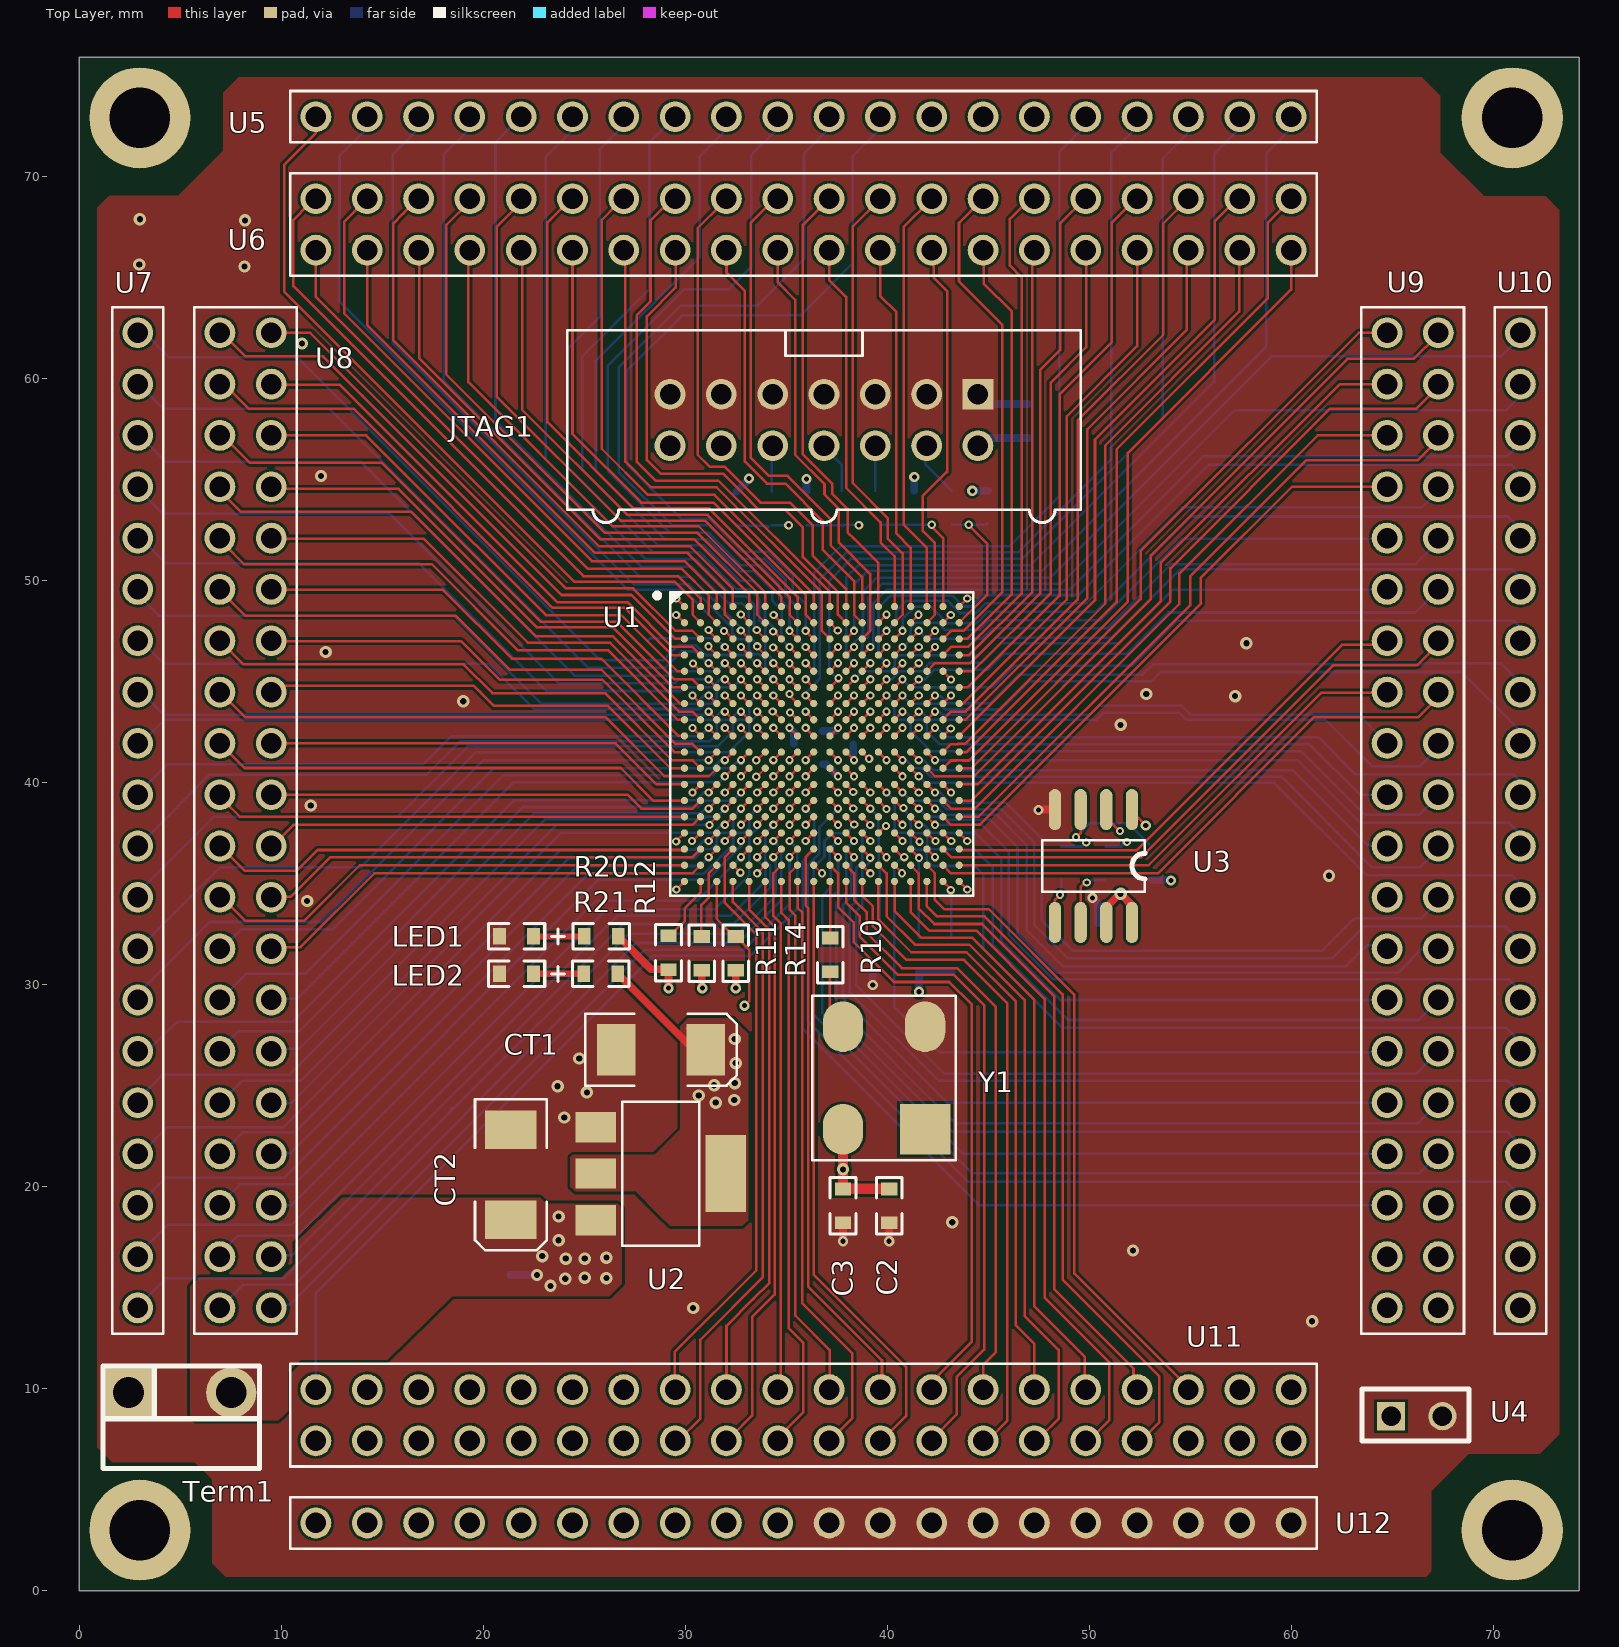
[diagram p0: Top Layer view]
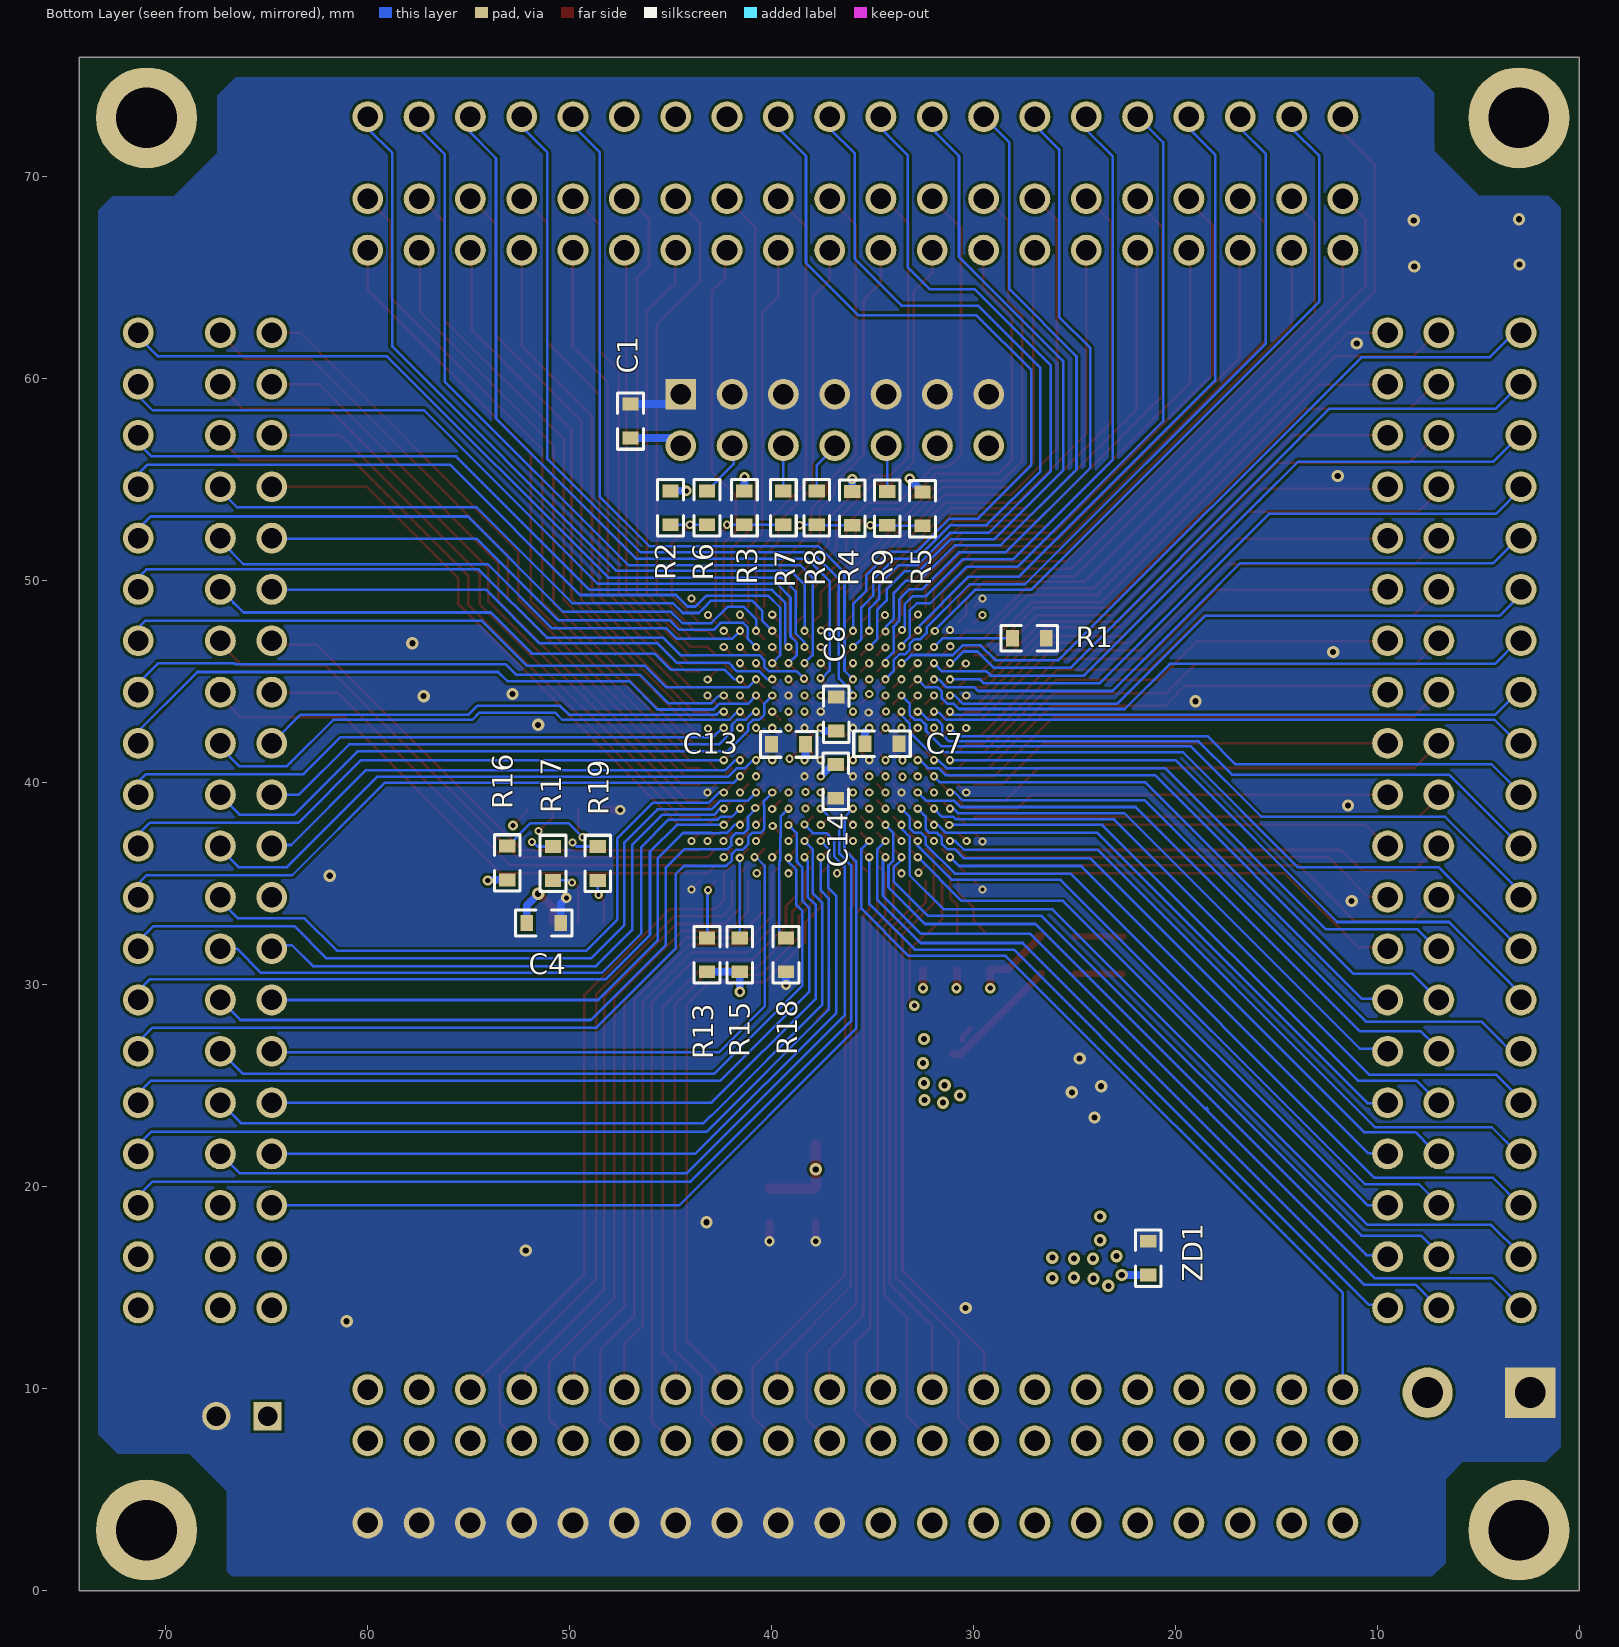
[diagram p1: Bottom Layer view, seen from below]
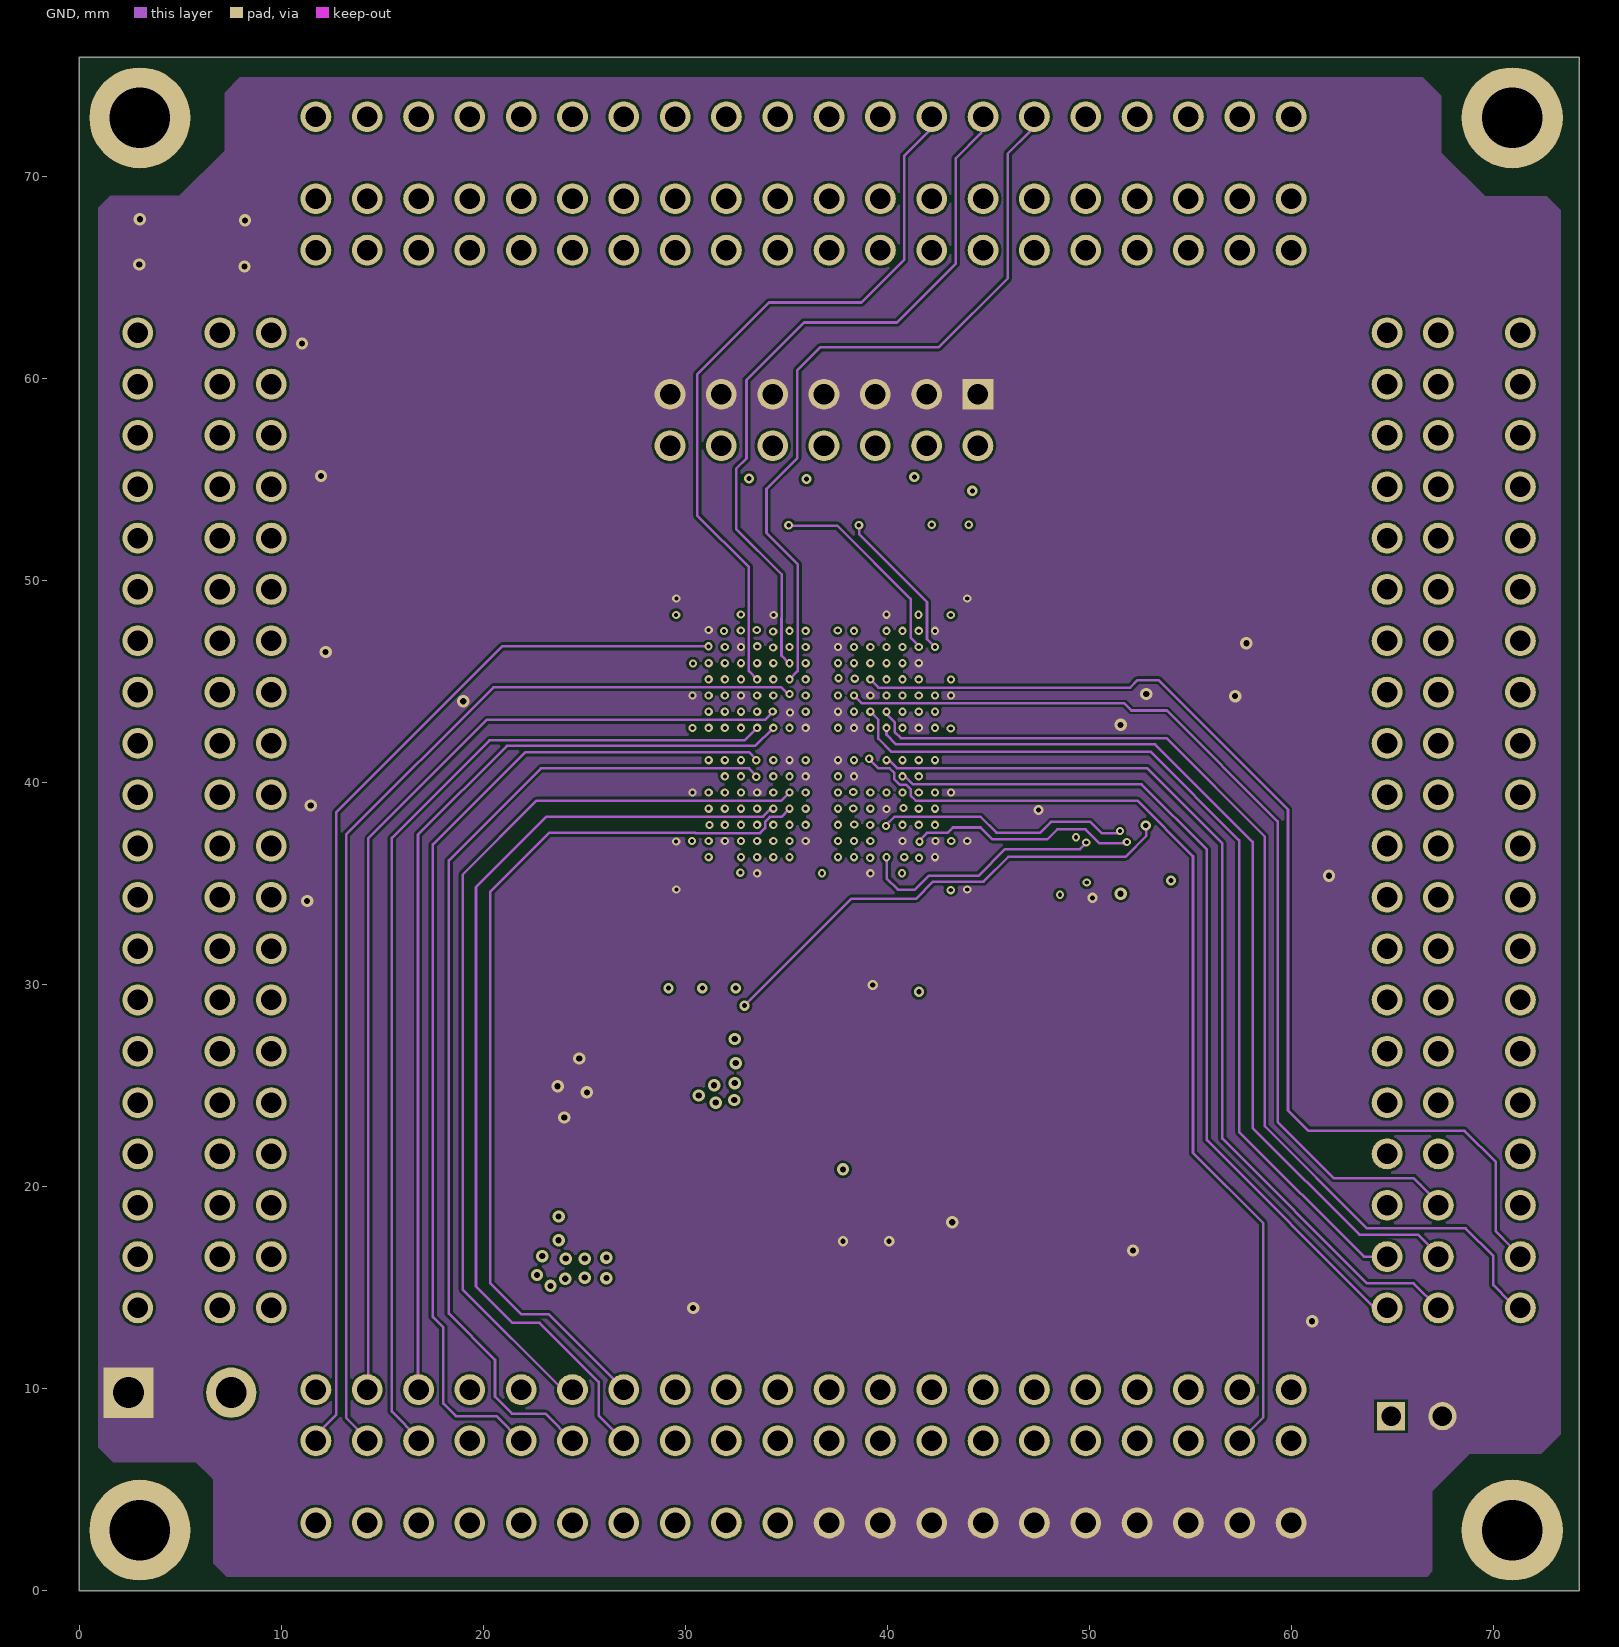
[diagram p2: GND]
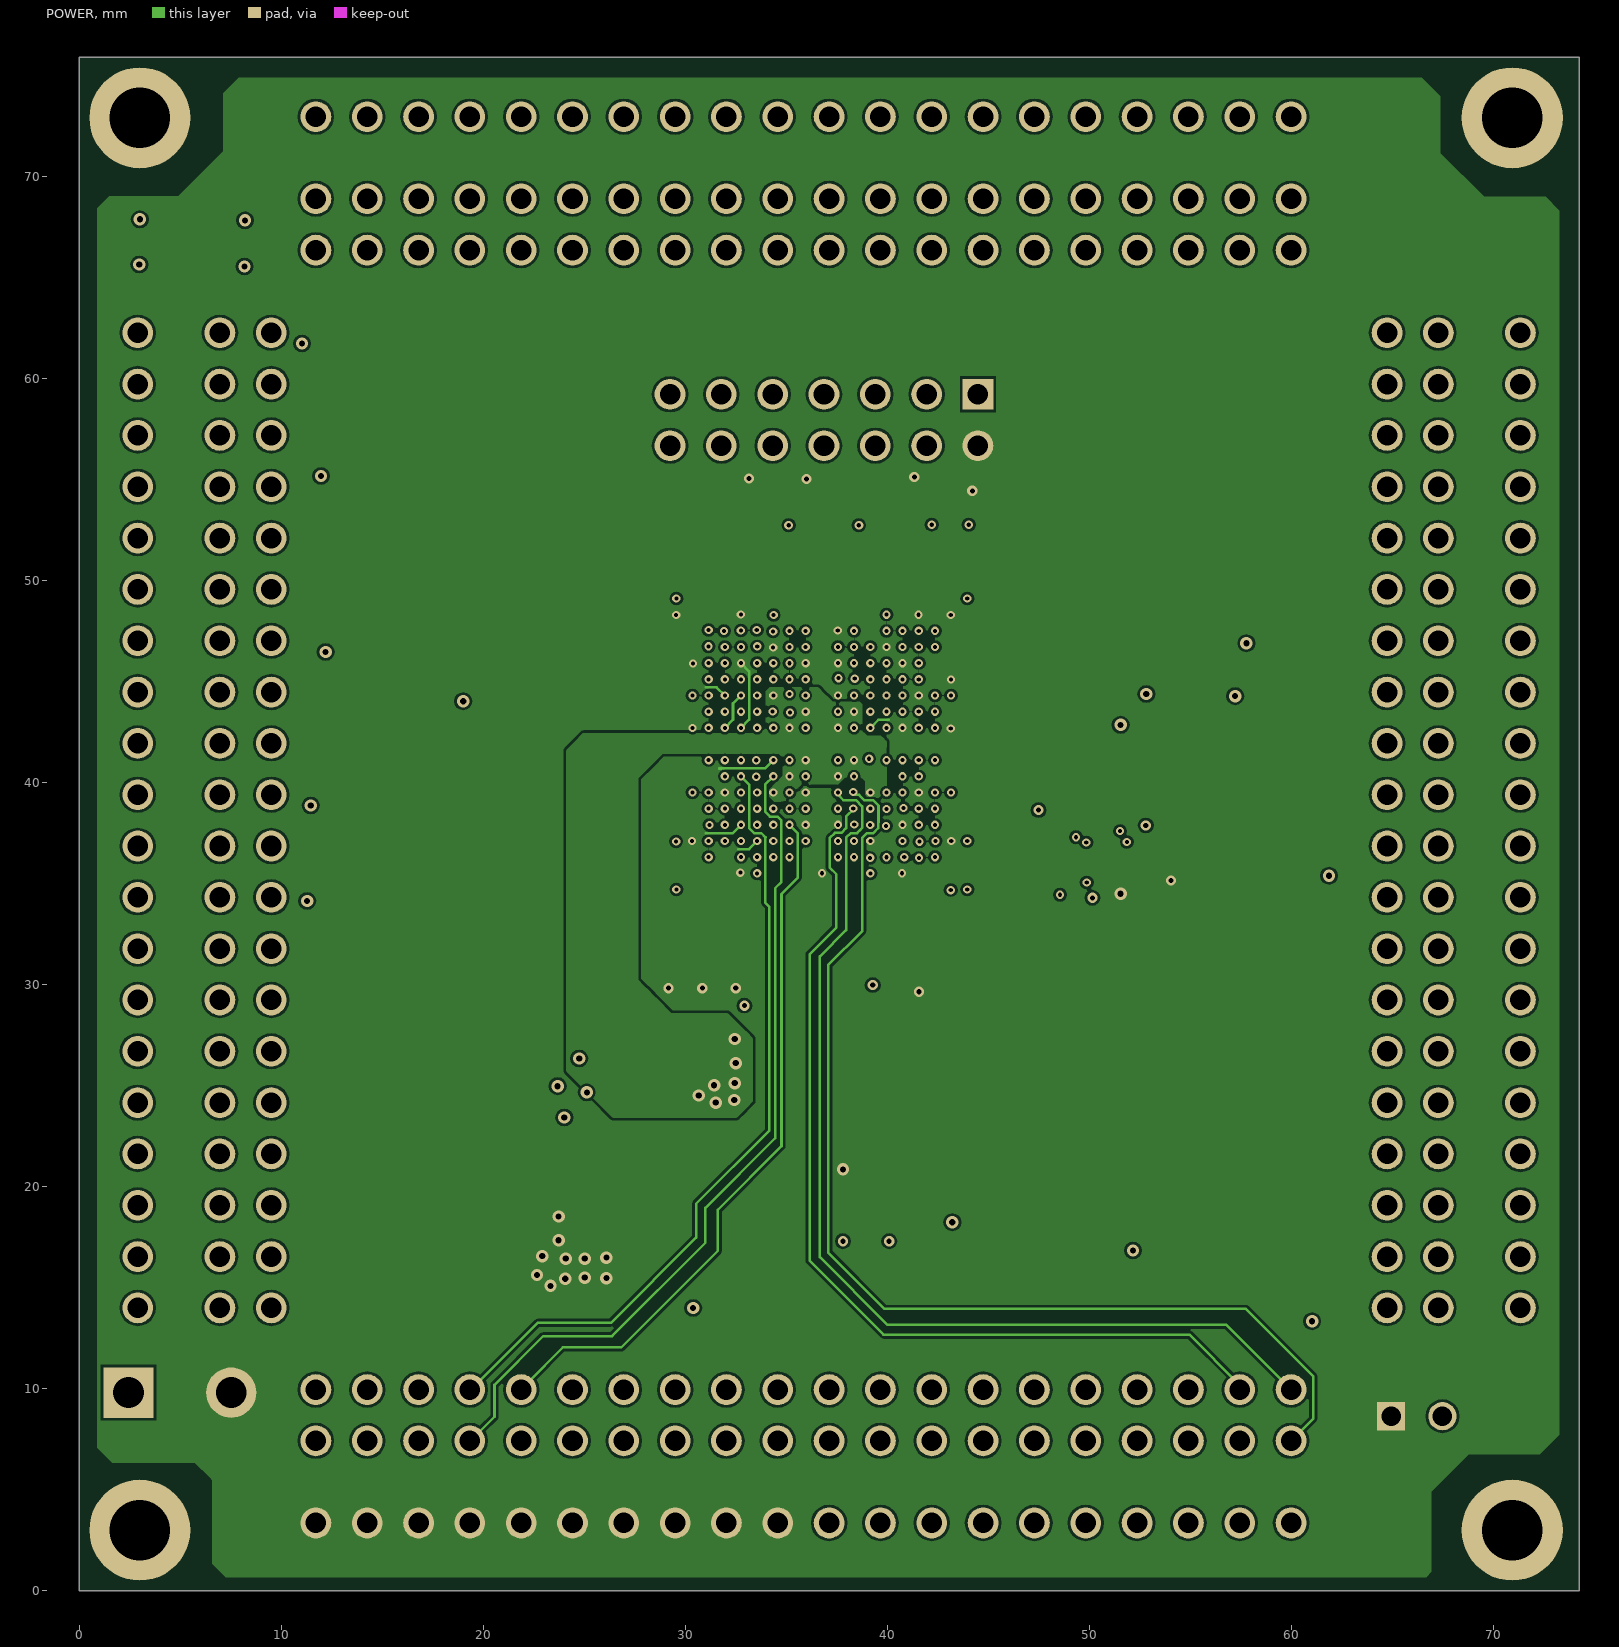
[diagram p3: POWER]
# Altium PCB MISC103828.PcbDoc (part 1 of 4)
Units mm, origin at the board's own origin, x right, y up, seen from the top; angles counter-clockwise.
Board outline 74.24 x 75.89 mm, 4 copper layers (Top Layer, GND, POWER, Bottom Layer); 49 components, 246 nets, 670 pads, 283 vias.

## Layer stack, top to bottom (the 12.6 mil dielectric is the usual default, probably not edited)
Top Layer: signal copper 0.0356
Dielectric: core 0.32, FR-4, Dk 4.8
GND: signal copper 0.0356
Dielectric: prepreg 0.32, FR-4, Dk 4.8
POWER: signal copper 0.0356
Dielectric: core 0.32, FR-4, Dk 4.8
Bottom Layer: signal copper 0.0356

## Board outline
0,0 0,75.889 74.244,75.889 74.244,0

## Design rules (kind name [scope] priority, off if disabled: settings)
Clearance [All] p1: gap=0.127
FabricationTestPointUsage TestPointUsage [All] p1: valid=0 allowmultiple=FALSE
FabricationTestpoint Testpoint [(IsPad And (OnTopLayer Or OnBottomLayer))] p1: side=3 testpointundercomponent=TRUE minsize=1.016 maxsize=2.54 preferedsize=1.524 minholesize=0 maxholesize=1.016 preferedholesize=0.813 testpointgrid=0.025 allowsidetop=TRUE allowsidebottom=TRUE usegrid=TRUE gridtolerance=0
HoleSize [All] p1: absolutevalues=TRUE maxlimit=12.7 minlimit=0.025 maxpercent=80.000 minpercent=20.000
HoleToHoleClearance [All] p1: gap=0.152 allowstackedmicrovias=TRUE
MinimumSolderMaskSliver [All] p1: minsoldermaskwidth=0.152
PolygonConnect PolygonConnect_1 [All vs isvia] p1: connectstyle=Direct reliefconductorwidth=0.254 reliefentries=4 polygonreliefangle="90 Angle"
PolygonConnect [All] p2: connectstyle=Direct reliefconductorwidth=0.254 reliefentries=4 polygonreliefangle="90 Angle"
RoutingVias [All] p1: holewidth=0.254 width=0.508 viastyle="Through Hole" minholewidth=0.203 minwidth=0.406 maxholewidth=0.508 maxwidth=0.762
SilkToSilkClearance [All] p1: silktosilkclearance=0
SilkscreenOverComponentPads [All] p1: minsilkscreentomaskgap=0
SolderMaskExpansion [All] p1: expansion=0.102
Width [All] p1: maxlimit=0.508 minlimit=0.127 preferedwidth=0.127 minimp=50.000000 maximp=50.000000 favimp=50.000000
21 further rules are at their usual default settings.

## Components (designator, comment, footprint, x,y, rotation, side; value= is the part's Value field where it differs from the comment)
C1 "0.1u" 0603 46.965,58.725 r270 bottom
C2 "0.1uF" 0603 40.081,18.212 r90 top
C3 "0.1uF" 0603 37.795,18.212 r90 top
C4 "0.1u" 0603 52.095,33.045 r180 bottom
C7 "0.1uF" 0603 33.68,41.91 r0 bottom
C8 "0.1uF" 0603 36.779,44.221 r270 bottom
C13 "0.1uF" 0603 39.98,41.885 r180 bottom
C14 "0.1uF" 0603 36.805,39.218 r90 bottom
CT1 "22u/10V" 7227 26.543,26.772 r0 top
CT2 "22u/10V" 7227 21.361,22.835 r270 top
JTAG1 "JTAG" IDC14S 44.475,59.207 r180 top
LED1 "LED" DIODE_2 22.479,32.385 r180 top
LED2 "LED" DIODE_2 22.479,30.531 r180 top
R1 "51" 0603 26.391,47.142 r0 bottom
R2 "10k" 0603 44.983,54.432 r270 bottom
R3 "10k" 0603 41.326,54.432 r270 bottom
R4 "10k" 0603 35.992,54.407 r270 bottom
R5 "10k" 0603 32.512,54.381 r270 bottom
R6 "51" 0603 43.18,52.756 r90 bottom
R7 "51" 0603 39.395,52.756 r90 bottom
R8 "51" 0603 37.744,52.756 r90 bottom
R9 "51" 0603 34.265,52.73 r90 bottom
R10 "22" 0603 37.16,30.632 r90 top
R11 "4.7k" 0603 30.81,30.709 r90 top
R12 "4.7k" 0603 29.159,30.734 r90 top
R13 "4.7k" 0603 43.18,30.632 r90 bottom
R14 "4.7k" 0603 32.487,30.709 r90 top
R15 "4.7k" 0603 41.554,30.632 r90 bottom
R16 "4.7k" 0603 53.061,36.855 r270 bottom
R17 "22" 0603 50.8,36.83 r270 bottom
R18 "22" 0603 39.268,30.632 r90 bottom
R19 "22" 0603 48.59,36.83 r270 bottom
R20 "2k" 0603 24.994,32.385 r0 top
R21 "2k" 0603 24.968,30.531 r0 top
Term1 "Phonix Connector 2p" PhonixCon2P 2.438,9.804 r0 top
U1 "XC6SLX9-CSG324" CSG324 36.747,41.903 r0 top
U2 "LM1117-1.2V" SOT223 25.552,22.936 r270 top
U3 "M25P80" M25P16_SO-8 52.095,38.659 r270 top
U4 "TP2" TP2 64.922,8.636 r0 top
U5 "TP20_2.54mm" TP20_2.54mm 11.709,72.949 r0 top
U6 "TP20*2_2.54mm" TP20*2_2.54mm 11.709,66.345 r0 top
U7 "TP20_2.54mm" TP20_2.54mm 2.896,62.255 r270 top
U8 "TP20*2_2.54mm" TP20*2_2.54mm 6.96,62.255 r270 top
U9 "TP20*2_2.54mm" TP20*2_2.54mm 64.719,62.255 r270 top
U10 "TP20_2.54mm" TP20_2.54mm 71.323,62.255 r270 top
U11 "TP20*2_2.54mm" TP20*2_2.54mm 11.709,7.417 r0 top
U12 "TP20_2.54mm" TP20_2.54mm 11.709,3.353 r0 top
Y1 "30MHz-3.3V" OSC-SO4 41.859,22.835 r90 top
ZD1 "T3V3S5" 0603 21.336,17.297 r270 bottom

## Footprints (in the part's own frame and the unit in brackets; to place one, negate y for a bottom-side part, rotate by r counter-clockwise, add the part's x,y. Pads: shape width x height; smd on the part's side, far side on the other; paste and mask are expansions set on the pad)
0603 [mil]
  rect 25x32 smd: 1(0,0) 2(66,0)
  silkscreen extent -22,-25 88,25
7227 [mil]
  rect 75x100 smd: 1(176,0) 2(1,0)
  silkscreen extent -59,-70 236,70
CSG324 [mm] "BGA, 324-Leads, Body 15x15mm, Pitch 0.8mm"
  round 0.36 smd: A1(-6.8,6.8) A2(-6,6.8) A3(-5.2,6.8) A4(-4.4,6.8) A5(-3.6,6.8) A6(-2.8,6.8) A7(-2,6.8) A8(-1.2,6.8) A9(-0.4,6.8) A10(0.4,6.8) A11(1.2,6.8) A12(2,6.8) A13(2.8,6.8) A14(3.6,6.8) A15(4.4,6.8) A16(5.2,6.8) A17(6,6.8) A18(6.8,6.8) B1(-6.8,6) B2(-6,6) B3(-5.2,6) B4(-4.4,6) B5(-3.6,6) B6(-2.8,6) B7(-2,6) B8(-1.2,6) B9(-0.4,6) B10(0.4,6) B11(1.2,6) B12(2,6) B13(2.8,6) B14(3.6,6) B15(4.4,6) B16(5.2,6) B17(6,6) B18(6.8,6) C1(-6.8,5.2) C2(-6,5.2) C3(-5.2,5.2) C4(-4.4,5.2) C5(-3.6,5.2) C6(-2.8,5.2) C7(-2,5.2) C8(-1.2,5.2) C9(-0.4,5.2) C10(0.4,5.2) C11(1.2,5.2) C12(2,5.2) C13(2.8,5.2) C14(3.6,5.2) C15(4.4,5.2) C16(5.2,5.2) C17(6,5.2) C18(6.8,5.2) D1(-6.8,4.4) D2(-6,4.4) D3(-5.2,4.4) D4(-4.4,4.4) D5(-3.6,4.4) D6(-2.8,4.4) D7(-2,4.4) D8(-1.2,4.4) D9(-0.4,4.4) D10(0.4,4.4) D11(1.2,4.4) D12(2,4.4) D13(2.8,4.4) D14(3.6,4.4) D15(4.4,4.4) D16(5.2,4.4) D17(6,4.4) D18(6.8,4.4) E1(-6.8,3.6) E2(-6,3.6) E3(-5.2,3.6) E4(-4.4,3.6) E5(-3.6,3.6) E6(-2.8,3.6) E7(-2,3.6) E8(-1.2,3.6) E9(-0.4,3.6) E10(0.4,3.6) E11(1.2,3.6) E12(2,3.6) E13(2.8,3.6) E14(3.6,3.6) E15(4.4,3.6) E16(5.2,3.6) E17(6,3.6) E18(6.8,3.6) F1(-6.8,2.8) F2(-6,2.8) F3(-5.2,2.8) F4(-4.4,2.8) F5(-3.6,2.8) F6(-2.8,2.8) F7(-2,2.8) F8(-1.2,2.8) F9(-0.4,2.8) F10(0.4,2.8) F11(1.2,2.8) F12(2,2.8) F13(2.8,2.8) F14(3.6,2.8) F15(4.4,2.8) F16(5.2,2.8) F17(6,2.8) F18(6.8,2.8) G1(-6.8,2) G2(-6,2) G3(-5.2,2) G4(-4.4,2) G5(-3.6,2) G6(-2.8,2) G7(-2,2) G8(-1.2,2) G9(-0.4,2) G10(0.4,2) G11(1.2,2) G12(2,2) G13(2.8,2) G14(3.6,2) G15(4.4,2) G16(5.2,2) G17(6,2) G18(6.8,2) H1(-6.8,1.2) H2(-6,1.2) H3(-5.2,1.2) H4(-4.4,1.2) H5(-3.6,1.2) H6(-2.8,1.2) H7(-2,1.2) H8(-1.2,1.2) H9(-0.4,1.2) H10(0.4,1.2) H11(1.2,1.2) H12(2,1.2) H13(2.8,1.2) H14(3.6,1.2) H15(4.4,1.2) H16(5.2,1.2) H17(6,1.2) H18(6.8,1.2) J1(-6.8,0.4) J2(-6,0.4) J3(-5.2,0.4) J4(-4.4,0.4) J5(-3.6,0.4) J6(-2.8,0.4) J7(-2,0.4) J8(-1.2,0.4) J9(-0.4,0.4) J10(0.4,0.4) J11(1.2,0.4) J12(2,0.4) J13(2.8,0.4) J14(3.6,0.4) J15(4.4,0.4) J16(5.2,0.4) J17(6,0.4) J18(6.8,0.4) K1(-6.8,-0.4) K2(-6,-0.4) K3(-5.2,-0.4) K4(-4.4,-0.4) K5(-3.6,-0.4) K6(-2.8,-0.4) K7(-2,-0.4) K8(-1.2,-0.4) K9(-0.4,-0.4) K10(0.4,-0.4) K11(1.2,-0.4) K12(2,-0.4) K13(2.8,-0.4) K14(3.6,-0.4) K15(4.4,-0.4) K16(5.2,-0.4) K17(6,-0.4) K18(6.8,-0.4) L1(-6.8,-1.2) L2(-6,-1.2) L3(-5.2,-1.2) L4(-4.4,-1.2) L5(-3.6,-1.2) L6(-2.8,-1.2) L7(-2,-1.2) L8(-1.2,-1.2) L9(-0.4,-1.2) L10(0.4,-1.2) L11(1.2,-1.2) L12(2,-1.2) L13(2.8,-1.2) L14(3.6,-1.2) L15(4.4,-1.2) L16(5.2,-1.2) L17(6,-1.2) L18(6.8,-1.2) M1(-6.8,-2) M2(-6,-2) M3(-5.2,-2) M4(-4.4,-2) M5(-3.6,-2) M6(-2.8,-2) M7(-2,-2) M8(-1.2,-2) M9(-0.4,-2) M10(0.4,-2) M11(1.2,-2) M12(2,-2) M13(2.8,-2) M14(3.6,-2) M15(4.4,-2) M16(5.2,-2) M17(6,-2) M18(6.8,-2) N1(-6.8,-2.8) N2(-6,-2.8) N3(-5.2,-2.8) N4(-4.4,-2.8) N5(-3.6,-2.8) N6(-2.8,-2.8) N7(-2,-2.8) N8(-1.2,-2.8) N9(-0.4,-2.8) N10(0.4,-2.8) N11(1.2,-2.8) N12(2,-2.8) N13(2.8,-2.8) N14(3.6,-2.8) N15(4.4,-2.8) N16(5.2,-2.8) N17(6,-2.8) N18(6.8,-2.8) P1(-6.8,-3.6) P2(-6,-3.6) P3(-5.2,-3.6) P4(-4.4,-3.6) P5(-3.6,-3.6) P6(-2.8,-3.6) P7(-2,-3.6) P8(-1.2,-3.6) P9(-0.4,-3.6) P10(0.4,-3.6) P11(1.2,-3.6) P12(2,-3.6) P13(2.8,-3.6) P14(3.6,-3.6) P15(4.4,-3.6) P16(5.2,-3.6) P17(6,-3.6) P18(6.8,-3.6) R1(-6.8,-4.4) R2(-6,-4.4) R3(-5.2,-4.4) R4(-4.4,-4.4) R5(-3.6,-4.4) R6(-2.8,-4.4) R7(-2,-4.4) R8(-1.2,-4.4) R9(-0.4,-4.4) R10(0.4,-4.4) R11(1.2,-4.4) R12(2,-4.4) R13(2.8,-4.4) R14(3.6,-4.4) R15(4.4,-4.4) R16(5.2,-4.4) R17(6,-4.4) R18(6.8,-4.4) T1(-6.8,-5.2) T2(-6,-5.2) T3(-5.2,-5.2) T4(-4.4,-5.2) T5(-3.6,-5.2) T6(-2.8,-5.2) T7(-2,-5.2) T8(-1.2,-5.2) T9(-0.4,-5.2) T10(0.4,-5.2) T11(1.2,-5.2) T12(2,-5.2) T13(2.8,-5.2) T14(3.6,-5.2) T15(4.4,-5.2) T16(5.2,-5.2) T17(6,-5.2) T18(6.8,-5.2) U1(-6.8,-6) U2(-6,-6) U3(-5.2,-6) U4(-4.4,-6) U5(-3.6,-6) U6(-2.8,-6) U7(-2,-6) U8(-1.2,-6) U9(-0.4,-6) U10(0.4,-6) U11(1.2,-6) U12(2,-6) U13(2.8,-6) U14(3.6,-6) U15(4.4,-6) U16(5.2,-6) U17(6,-6) U18(6.8,-6) V1(-6.8,-6.8) V2(-6,-6.8) V3(-5.2,-6.8) V4(-4.4,-6.8) V5(-3.6,-6.8) V6(-2.8,-6.8) V7(-2,-6.8) V8(-1.2,-6.8) V9(-0.4,-6.8) V10(0.4,-6.8) V11(1.2,-6.8) V12(2,-6.8) V13(2.8,-6.8) V14(3.6,-6.8) V15(4.4,-6.8) V16(5.2,-6.8) V17(6,-6.8) V18(6.8,-6.8)
  silkscreen extent -8.27,-7.5 7.5,7.5
DIODE_2 [mil]
  rect 25x32 smd: A(0,0) K(66,0)
  silkscreen extent -60,-25 88,25
IDC14S [mil]
  rect 60x60 hole 40: 1(0,0)
  round 60 hole 40: 2(0,100) 3(100,0) 4(100,100) 5(200,0) 6(200,100) 7(300,0) 8(300,100) 9(400,0) 10(400,100) 11(500,0) 12(500,100) 13(600,0) 14(600,100)
  silkscreen extent -200,-125 800,250
M25P16_SO-8 [mil]
  oval 80x24 smd: 1(0,0) 2(0,-50) 3(0,-100) 4(0,-150) 5(220,-150) 6(220,-100) 7(220,-50) 8(220,0)
  silkscreen extent 60,-175 160,25
OSC-SO4 [mm]
  rect 2.5x2.5 smd: 1(0,0)
  oval 2.5x2 smd: 2(5.08,0) 3(5.08,4.064) 4(0,4.064)
  silkscreen extent -1.52,-1.52 6.6,5.59
PhonixCon2P [mil]
  rect 98x98 hole 60: 1(0,0)
  round 98 hole 60: 2(200,0)
  silkscreen extent -50,-148 255,52
SOT223 [mil]
  rect 59x79 smd: 1(0,0) 2(90,0) 3(181,0)
  rect 150x79 smd: 2(90,254)
  silkscreen extent -49,52 231,202
TP2 [mil]
  rect 55x55 hole 38: 1(0,0)
  round 55 hole 38: 2(100,0)
  silkscreen extent -57,-48 152,53
TP20*2_2.54mm [mil]
  round 60 hole 40: 1(0,0) 2(0,100) 3(100,0) 4(100,100) 5(200,0) 6(200,100) 7(300,0) 8(300,100) 9(400,0) 10(400,100) 11(500,0) 12(500,100) 13(600,0) 14(600,100) 15(700,0) 16(700,100) 17(800,0) 18(800,100) 19(900,0) 20(900,100) 21(1000,0) 22(1000,100) 23(1100,0) 24(1100,100) 25(1200,0) 26(1200,100) 27(1300,0) 28(1300,100) 29(1400,0) 30(1400,100) 31(1500,0) 32(1500,100) 33(1600,0) 34(1600,100) 35(1700,0) 36(1700,100) 37(1800,0) 38(1800,100) 39(1900,0) 40(1900,100)
  silkscreen extent -50,-50 1950,150
TP20_2.54mm [mil]
  round 60 hole 40: 1(0,0) 2(100,0) 3(200,0) 4(300,0) 5(400,0) 6(500,0) 7(600,0) 8(700,0) 9(800,0) 10(900,0) 11(1000,0) 12(1100,0) 13(1200,0) 14(1300,0) 15(1400,0) 16(1500,0) 17(1600,0) 18(1700,0) 19(1800,0) 20(1900,0)
  silkscreen extent -50,-50 1950,50

## Part data
C1 C4: library part CAP, "Multilayer ceramic capacitor"
C2 C3 C7 C8 C13 C14: library part CAP, "Capacitor"
CT1 CT2: library part CAPACITOR, "Capacitor"
JTAG1: library part IDC14
R1 R2 R3 R4 R5 R6 R7 R8 R9 R10 R11 R12 R13 R14 R15 R16 R17 R18 R19 R20 R21: library part RES2
U1: library part XC6SLX25-CSG324
U2: library part 7810
Y1: library part OSCILLATOR
ZD1: library part "D Tunnel2", "Tunnel Diode - Dependent Source Model"

## Free pads (board coordinates)
  round 5 hole 3: 0(3,3) 0(3,72.889) 0(70.915,3) 0(70.915,72.889)

## Via types
v1: diameter 0.406, hole 0.203, Top Layer to Bottom Layer, 221 vias
v2: diameter 0.61, hole 0.305, Top Layer to Bottom Layer, 43 vias
v3: diameter 0.508, hole 0.254, Top Layer to Bottom Layer, 16 vias
v4: diameter 0.432, hole 0.229, Top Layer to Bottom Layer, 3 vias

## Nets (pads, with @x,y where several pads share a name; then routed paths per layer and width w, separated by ;. In a path a pad name is that pad's centre, name@x,y a point inside that pad or via, vN(x,y) a via of type N, cw(c..) or ccw(c..) an arc to the next point about the centre after c; other vN are vias at no path point)
+1.2V: C7.2 C8.2 C13.2 C14.2 CT1.1 R21.2 U1.G7 U1.H9 U1.H11 U1.J8 U1.J10 U1.K9 U1.K11 U1.L8 U1.L10 U1.M7 U1.M12 U2.2 | length 16.5
  Top Layer w0.127: v1(34.347,39.503) U1.M7@34.747,39.903 ; v1(34.347,44.303) U1.G7@34.747,43.903 ; v1(35.147,40.303) U1.L8@35.547,40.703 ; v1(35.147,42.703) U1.J8@35.547,42.303 ; v1(35.947,41.103) U1.K9@36.347,41.503 ; v1(35.947,43.503) U1.H9@36.347,43.103 ; U1.L10@37.147,40.703 v1(37.547,40.303) ; U1.J10@37.147,42.303 v1(37.547,42.703) ; U1.K11@37.947,41.503 v1(38.347,41.103) ; U1.H11@37.947,43.103 v1(38.347,43.503) ; U1.M12@38.747,39.903 v1(39.147,39.503)
  Top Layer w0.254: CT1.1@30.137,27.826 30.531,27.432 CT1.1@30.531,27.229
  Top Layer w0.381: R21.2@26.645,30.531 30.632,26.543 CT1.1@31.013,26.543
  Bottom Layer w0.381: v1(35.147,42.703) 35.357,42.494 C7.2@35.357,41.91 ; C8.2@36.779,42.545 37.389,42.545 v1(37.547,42.703) ; C14.2@36.805,40.894 36.957,40.894 v1(37.547,40.303) ; C13.2@38.303,41.885 38.303,41.148 v1(38.347,41.103)
  other v2: 31.496,24.155 32.41,24.282 30.658,24.511 31.42,25.019 32.436,25.121 32.487,26.111 32.436,27.305
+3.3V: C1.2 C2.2 C3.2 C4.1 CT2.1 JTAG1.2 R2.1 R3.1 R4.1 R5.1 R11.1 R12.1 R13.1 R14.1 R15.1 R16.2 R20.2 Term1.2 U1.B1 U1.B5 U1.B10 U1.B15 U1.B17 U1.D7 U1.D13 U1.E2 U1.E5 U1.E9 U1.E10 U1.E14 U1.E17 U1.G4 U1.G10 U1.G15 U1.J2 U1.J5 U1.J12 U1.J14 U1.J17 U1.K7 U1.M4 U1.M9 U1.M15 U1.P5 U1.P9 U1.P10 U1.P14 U1.R2 U1.R6 U1.R12 U1.R17 U1.U4 U1.U9 U1.U14 U2.3 U3.7 U3.8 U4.1 U12.1 U12.2 U12.3 U12.4 U12.5 U12.6 U12.7 U12.8 U12.9 U12.10 Y1.4 ZD1.2 | length 57.4
  Top Layer w0.127: v1(29.54,48.285) 29.565,48.285 U1.B1@29.947,47.903 ; v1(30.328,37.109) 30.347,37.109 30.363,37.125 30.369,37.125 U1.R2@30.747,37.503 ; v1(30.353,42.697) U1.J2@30.747,42.303 ; v1(30.369,45.888) 30.369,45.882 U1.E2@30.747,45.503 ; v1(31.947,39.503) U1.M4@32.347,39.903 ; v1(31.947,44.303) U1.G4@32.347,43.903 ; U1.U4@32.347,35.903 v1(32.715,35.535) ; v1(32.741,48.311) 32.766,48.285 U1.B5@33.147,47.903 ; v1(32.747,37.903) U1.P5@33.147,38.303 ; v1(32.747,42.703) U1.J5@33.147,42.303 ; v1(32.747,45.903) U1.E5@33.147,45.503 ; v1(33.547,37.103) U1.R6@33.947,37.503 ; v1(34.347,41.103) U1.K7@34.747,41.503 ; v1@34.468,46.609 34.747,46.329 U1.D7@34.747,46.303 ; v1(35.947,37.903) U1.P9@36.347,38.303 ; v1(35.947,39.503) U1.M9@36.347,39.903 ; v1(35.947,45.903) U1.E9@36.347,45.503 ; U1.U9@36.347,35.903 36.744,35.506 v1(36.751,35.506) ; U1.P10@37.147,38.303 v1(37.547,37.903) ; U1.G10@37.147,43.903 v1(37.547,44.303) ; U1.E10@37.147,45.503 v1(37.547,45.903) ; U1.B10@37.147,47.903 37.531,47.52 v1(37.538,47.52) ; U1.R12@38.747,37.503 v1(39.147,37.103) ; U1.J12@38.747,42.303 v1(39.147,42.703) ; U1.D13@39.547,46.303 v1(39.947,46.703) ; U1.U14@40.347,35.903 40.716,35.535 v1(40.716,35.509) ; U1.P14@40.347,38.303 v1(40.747,37.903) ; U1.J14@40.347,42.303 v1(40.747,42.703) ; U1.E14@40.347,45.503 v1(40.747,45.903) ; U1.M15@41.147,39.903 v1(41.547,39.503) ; U1.G15@41.147,43.903 v1(41.547,44.303) ; U1.B15@41.147,47.903 41.539,48.295 v1(41.539,48.301) ; U1.R17@42.747,37.503 43.145,37.106 v1(43.151,37.106) ; U1.J17@42.747,42.303 43.119,42.675 v1(43.126,42.675) ; U1.E17@42.747,45.503 43.144,45.107 v1(43.144,45.1) ; U1.B17@42.747,47.903 v1(43.129,48.285)
  Top Layer w0.381: R20.2@26.797,32.385 R20.2@26.67,32.385 28.296,30.759 R12.1@29.159,30.759 ; v3(29.159,29.82) R12.1@29.159,30.734 ; R11.1@30.81,30.709 30.81,29.82 v3(30.836,29.82) ; v3(32.487,29.82) R14.1@32.487,30.709 ; C3.2@37.795,19.964 C3.2@37.871,19.888 ; U3.7@50.825,33.071 50.825,33.833 v2@51.486,34.493 ; v2(51.537,34.493) 52.095,33.934 U3.8@52.095,33.071
  Top Layer w0.508: C3.2@37.795,19.964 Y1.4@37.795,22.073 ; C3.2@37.871,19.888 C2.2@40.081,19.888
  POWER w0.127: 31.013,37.497 32.341,37.497 v1(32.747,37.903) ; 31.013,44.704 31.547,44.704 v1(31.947,44.303) ; 31.674,40.691 31.778,40.691 31.784,40.697 33.941,40.697 v1(34.347,41.103) ; 32.614,36.703 33.147,36.703 v1(33.547,37.103) ; v1(32.747,42.703) 33.154,43.11 33.154,44.983 ; v1(32.747,45.903) 33.154,45.497 33.154,44.983 ; 33.154,45.11 33.154,44.983 ; v1(39.147,42.703) 39.548,43.104 40.056,43.104
  Bottom Layer w0.127: v1@30.328,42.697 v1(30.353,42.697) ; v1@32.715,48.235 32.766,48.285 v1(32.741,48.311) ; v1@43.129,45.085 v1(43.144,45.1)
  Bottom Layer w0.381: ZD1.2@21.336,15.621 v2@22.479,15.621 ; R5.1@32.512,54.381 33.147,55.016 v3(33.147,55.042) ; R4.1@35.992,54.407 v3(35.992,55.016) ; R3.1@41.326,54.432 v3(41.326,55.118) ; v3(41.554,29.642) R15.1@41.554,30.632 ; R15.1@41.758,30.582 41.808,30.632 R13.1@43.18,30.632 ; v3(44.196,54.432) R2.1@44.983,54.432 ; JTAG1.2@44.552,56.667 44.933,57.048 C1.2@46.965,57.048 ; v2@51.562,34.442 52.095,33.909 C4.1@52.095,33.045 ; R16.2@53.061,35.179 54,35.179 v3(54.026,35.154)
  other v1: 34.341,46.685
  other v2: 23.317,15.088 24.054,15.443 26.086,15.469 25.019,15.494 22.657,15.621 24.079,16.434 25.019,16.434 26.086,16.485 22.911,16.561 23.724,17.348 23.724,18.517 37.795,20.853
F_A2: U1.A2 U6.2 | length 31.6
  Top Layer w0.127: U6.2@11.659,68.605 11.354,68.605 10.592,67.843 10.592,64.567 24.943,50.216 29.642,50.216 30.747,49.11 U1.A2@30.747,48.703
F_A3: U1.A3 U6.4 | length 31.1
  Top Layer w0.127: U6.4@14.211,68.923 U6.4@14.275,68.986 ; U6.4@14.249,68.885 13.106,67.742 13.106,63.221 25.375,50.952 29.947,50.952 31.547,49.352 U1.A3@31.547,48.703
F_A4: U1.A4 U6.6 | length 30.3
  Top Layer w0.127: 16.078,68.199 16.027,68.148 ; U6.6@16.688,68.885 16.688,68.809 16.027,68.148 ; U1.A4@32.347,48.703 32.347,49.568 30.226,51.689 25.73,51.689 15.545,61.874 15.545,67.666 16.027,68.148
F_A5: U1.A5 U6.5 | length 27.1
  Top Layer w0.127: U6.5@16.789,66.345 16.815,66.319 16.815,61.011 25.781,52.045 30.429,52.045 33.147,49.326 U1.A5@33.147,48.703
F_A6: U1.A6 U6.7 | length 26
  Top Layer w0.127: U6.7@19.38,66.04 19.253,65.913 19.253,59.817 26.391,52.68 30.658,52.68 33.947,49.39 U1.A6@33.947,48.703
F_A7: U1.A7 U6.10 | length 28.7
  Top Layer w0.127: U6.10@21.844,68.656 21.819,68.656 20.65,67.488 20.65,59.106 26.797,52.959 30.963,52.959 34.747,49.174 U1.A7@34.747,48.703
F_A8: U1.A8 U6.12 | length 28.1
  Top Layer w0.127: U6.12@24.409,68.885 24.333,68.885 23.165,67.716 23.165,57.836 27.432,53.569 31.166,53.569 35.547,49.187 U1.A8@35.547,48.703
F_A9: U1.A9 U6.14 | length 26.5
  Top Layer w0.127: U6.14@26.619,68.631 26.619,68.605 25.857,67.843 25.857,56.515 28.143,54.229 31.445,54.229 36.347,49.327 U1.A9@36.347,48.703
F_A10: U1.A10 U6.16 | length 26.5
  Top Layer w0.127: U6.16@29.235,68.758 29.21,68.758 28.27,67.818 28.27,63.805 27.584,63.119 27.584,55.88 28.524,54.94 31.623,54.94 37.147,49.416 U1.A10@37.147,48.703
F_A11: U1.A11 U6.18 | length 24.8
  Top Layer w0.127: U6.18@31.826,68.656 30.607,67.437 30.607,56.21 31.191,55.626 31.934,55.626 33.712,53.848 35.179,53.848 36.297,52.73 36.297,51.232 37.947,49.581 U1.A11@37.947,48.703
F_A12: U1.A12 U6.20 | length 23.4
  Top Layer w0.127: U6.20@34.341,68.859 34.341,68.809 33.223,67.691 33.223,56.083 34.138,55.169 35.052,55.169 37.186,53.035 37.186,51.74 38.747,50.178 U1.A12@38.747,48.703
F_A13: U1.A13 U6.22 | length 22.4
  Top Layer w0.127: U6.22@37.109,68.885 35.814,67.589 35.814,56.236 37.262,54.788 37.262,54.305 38.024,53.543 38.024,52.375 38.354,52.045 ; 38.291,52.108 38.354,52.045 ; U1.A13@39.547,48.703 39.547,50.851 38.354,52.045
F_A14: U1.A14 U6.21 | length 19
  Top Layer w0.127: U6.21@37.109,66.345 37.109,64.872 37.948,64.033 37.948,54.585 39.662,52.87 39.662,51.88 40.347,51.194 U1.A14@40.347,48.703
F_A15: U1.A15 U6.23 | length 18.3
  Top Layer w0.127: U6.23@39.649,66.345 39.649,64.059 40.437,63.271 40.437,52.324 41.147,51.613 U1.A15@41.147,48.703
F_A16: U1.A16 U6.26 | length 21.2
  Top Layer w0.127: U1.A16@41.947,48.703 41.947,51.601 40.792,52.756 40.792,67.488 U6.26@42.189,68.885
F_B2: U1.B2 U5.1 | length 37.2
  Top Layer w0.127: U5.1@11.709,72.949 11.709,72.136 10.135,70.561 10.135,64.287 24.486,49.936 29.464,49.936 30.352,49.049 30.352,48.299 U1.B2@30.747,47.903
F_B3: U1.B3 U6.1 | length 29.4
  Top Layer w0.127: U6.1@11.709,66.345 11.709,64.033 25.171,50.571 29.82,50.571 31.152,49.239 31.152,48.299 U1.B3@31.547,47.903
F_B4: U1.B4 U6.3 | length 28.2
  Top Layer w0.127: U6.3@14.275,65.938 14.249,65.913 14.249,62.636 25.527,51.359 30.099,51.359 31.952,49.506 31.952,48.299 U1.B4@32.347,47.903
F_B6: U1.B6 U6.8 | length 30.7
  Top Layer w0.127: U6.8@19.329,68.885 19.329,68.758 18.161,67.589 18.161,60.198 26.01,52.349 30.593,52.349 33.553,49.389 33.553,48.87 33.552,48.868 33.552,48.299 U1.B6@33.947,47.903
F_B8: U1.B8 U6.9 | length 26.4
  Top Layer w0.127: 21.92,65.253 21.92,65.176 ; U6.9@21.996,66.243 21.92,66.167 21.92,65.176 ; U1.B8@35.547,47.903 35.152,48.299 35.152,49.188 31.101,53.238 27.127,53.238 21.92,58.445 21.92,65.176
F_B9: U1.B9 U6.11 | length 25.5
  Top Layer w0.127: U6.11@24.409,66.345 24.409,57.252 27.813,53.848 31.394,53.848 35.943,49.299 35.943,48.307 U1.B9@36.347,47.903
F_B11: U1.B11 U6.15 | length 25.4
  Top Layer w0.127: U6.15@29.566,65.964 29.515,65.913 29.515,64.491 28.092,63.068 28.092,55.956 28.778,55.27 31.877,55.27 33.198,53.95 ; 33.172,53.95 33.604,53.518 34.925,53.518 35.814,52.629 35.814,51.156 37.543,49.426 37.543,48.307 U1.B11@37.947,47.903
F_B12: U1.B12 U6.17 | length 22.8
  Top Layer w0.127: U6.17@31.979,65.862 32.055,65.938 32.055,66.548 32.029,66.573 32.029,65.227 32.944,64.313 32.944,60.833 ; 32.944,60.909 32.944,60.833 ; U1.B12@38.747,47.903 38.351,48.299 38.351,49.964 36.792,51.524 36.792,52.946 34.95,54.788 34.036,54.788 32.944,55.88 32.944,60.833
F_B14: U1.B14 U6.24 | length 22.7
  Top Layer w0.127: U6.24@39.649,68.885 38.278,67.513 38.278,54.813 40.005,53.086 40.005,52.07 40.743,51.332 40.743,48.299 U1.B14@40.347,47.903
F_B16: U1.B16 U6.25 | length 20.8
  Top Layer w0.127: U1.B16@41.947,47.903 42.343,48.299 42.343,51.84 41.745,52.438 41.745,54.191 42.901,55.347 ; U6.25@42.113,65.862 42.139,65.888 42.139,66.523 42.291,66.675 42.291,64.973 42.951,64.313 42.951,55.347
F_C1: U1.C1 U8.1 | length 28.9
  Top Layer w0.127: U8.1@7.264,62.052 8.23,61.087 12.065,61.087 14.021,59.131 23.876,49.276 27.33,49.276 29.503,47.103 U1.C1@29.947,47.103
F_C2: U1.C2 U8.2 | length 27.5
  Top Layer w0.127: U8.2@9.5,62.255 11.43,62.255 24.079,49.606 27.407,49.606 29.505,47.507 30.343,47.507 U1.C2@30.747,47.103
F_C4: U1.C4 U5.2 | length 35.6
  Top Layer w0.127: v1(31.902,47.498) 31.928,47.498 31.927,47.499 31.927,47.503 31.947,47.503 U1.C4@32.347,47.103
  Bottom Layer w0.127: U5.2@14.249,72.365 12.878,70.993 12.878,63.805 27.153,49.53 29.921,49.53 31.947,47.503 31.927,47.503 31.927,47.499 31.928,47.498 v1(31.902,47.498)
F_C5: U1.C5 U5.4 | length 33.6
  Top Layer w0.127: v1@32.764,47.486 U1.C5@33.147,47.103
  Bottom Layer w0.127: U5.4@19.329,72.365 18.034,71.069 18.034,59.893 27.737,50.19 30.226,50.19 32.786,47.631 v1@32.786,47.508 ; v1(32.741,47.523) 32.766,47.498 32.791,47.498 32.791,47.508 v1@32.786,47.508